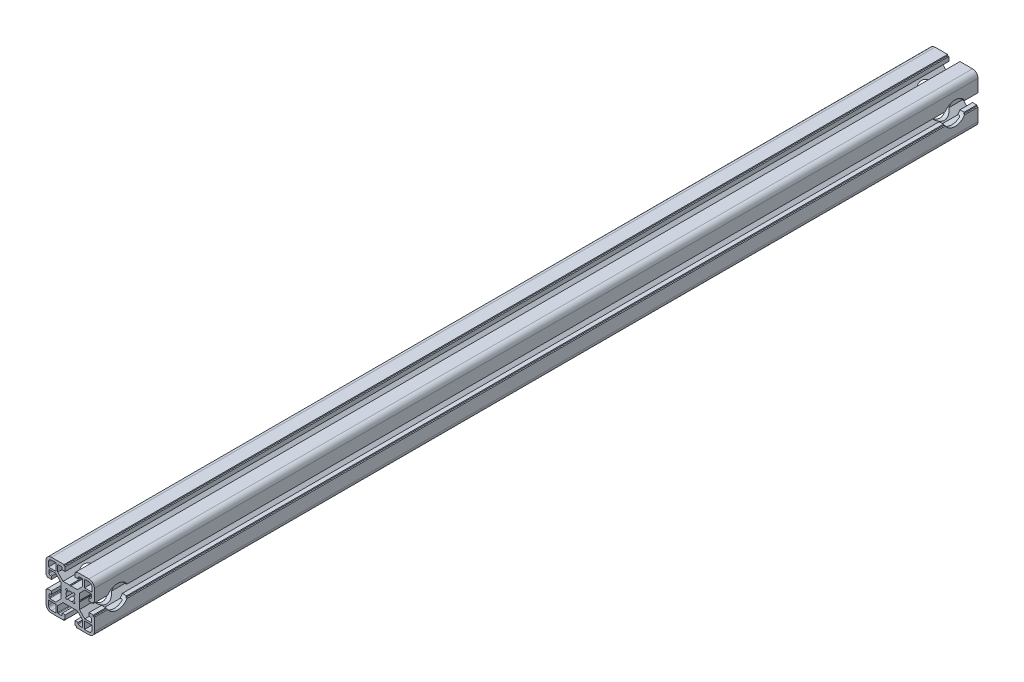
SolidWorks part; units mm, degrees
material "6061 GB/T6892-2006"
ref_plane "前视" through (0, 0, 0) normal (0, 0, 1) x (1, 0, 0)
ref_plane "上视" through (0, 0, 0) normal (0, 1, 0) x (1, 0, 0)
ref_plane "右视" through (0, 0, 0) normal (1, 0, 0) x (0, 0, -1)
sketch "草图1" plane through (0, 0, 0) normal (0, 0, 1) x (1, 0, 0)
  line L0 (-18.9995, -4.1003) -> (-18.9995, -5.1003)
  line L1 (-18.9995, -5.1003) -> (-19.9995, -5.1003)
  line L2 (-19.9995, -5.1003) -> (-19.9995, -15.5003)
  line L3 (-15.4995, -20.0003) -> (-5.0995, -20.0003)
  line L4 (-5.0995, -20.0003) -> (-5.0995, -19.0003)
  line L5 (-5.0995, -19.0003) -> (-4.0995, -19.0003)
  line L6 (-4.0995, -19.0003) -> (-4.0995, -15.5003)
  line L7 (-4.0995, -15.5003) -> (-6.5995, -15.5003)
  line L8 (-6.5995, -15.5003) -> (-6.5995, -16.5003)
  line L9 (-7.5995, -17.5003) -> (-9.7995, -17.5003)
  line L10 (-10.2995, -17.0003) -> (-10.2995, -11.9973)
  line L11 (-10.2995, -11.9973) -> (-5.9025, -7.6003)
  line L12 (-5.9025, -7.6003) -> (-0.5195, -7.6003)
  line L13 (-0.5195, -7.6003) -> (0.0005, -7.3003)
  line L14 (0.0005, -7.3003) -> (0.5195, -7.6003)
  line L15 (0.5195, -7.6003) -> (5.9035, -7.6003)
  line L16 (5.9035, -7.6003) -> (10.3005, -11.9973)
  line L17 (10.3005, -11.9973) -> (10.3005, -17.0003)
  line L18 (9.8005, -17.5003) -> (7.6005, -17.5003)
  line L19 (6.6005, -16.5003) -> (6.6005, -15.5003)
  line L20 (6.6005, -15.5003) -> (4.1005, -15.5003)
  line L21 (4.1005, -15.5003) -> (4.1005, -19.0003)
  line L22 (4.1005, -19.0003) -> (5.1005, -19.0003)
  line L23 (5.1005, -19.0003) -> (5.1005, -20.0003)
  line L24 (5.1005, -20.0003) -> (15.5005, -20.0003)
  line L25 (20.0005, -15.5003) -> (20.0005, -5.1003)
  line L26 (20.0005, -5.1003) -> (19.0005, -5.1003)
  line L27 (19.0005, -5.1003) -> (19.0005, -4.1003)
  line L28 (19.0005, -4.1003) -> (15.5005, -4.1003)
  line L29 (15.5005, -4.1003) -> (15.5005, -6.6003)
  line L30 (15.5005, -6.6003) -> (16.5005, -6.6003)
  line L31 (17.5005, -7.6003) -> (17.5005, -9.8003)
  line L32 (17.0005, -10.3003) -> (11.9975, -10.3003)
  line L33 (11.9975, -10.3003) -> (7.6005, -5.9033)
  line L34 (7.6005, -5.9033) -> (7.6005, -0.5203)
  line L35 (7.6005, -0.5203) -> (7.3005, -0.0003)
  line L36 (7.3005, -0.0003) -> (7.6005, 0.5197)
  line L37 (7.6005, 0.5197) -> (7.6005, 5.9027)
  line L38 (7.6005, 5.9027) -> (11.9975, 10.2997)
  line L39 (11.9975, 10.2997) -> (17.0005, 10.2997)
  line L40 (17.5005, 9.7997) -> (17.5005, 7.5997)
  line L41 (16.5005, 6.5997) -> (15.5005, 6.5997)
  line L42 (15.5005, 6.5997) -> (15.5005, 4.0997)
  line L43 (15.5005, 4.0997) -> (19.0005, 4.0997)
  line L44 (19.0005, 4.0997) -> (19.0005, 5.0997)
  line L45 (19.0005, 5.0997) -> (20.0005, 5.0997)
  line L46 (20.0005, 5.0997) -> (20.0005, 15.4997)
  line L47 (15.5005, 19.9997) -> (5.1005, 19.9997)
  line L48 (5.1005, 19.9997) -> (5.1005, 18.9997)
  line L49 (5.1005, 18.9997) -> (4.1005, 18.9997)
  line L50 (4.1005, 18.9997) -> (4.1005, 15.4997)
  line L51 (4.1005, 15.4997) -> (6.6005, 15.4997)
  line L52 (7.6005, 17.4997) -> (9.8005, 17.4997)
  line L53 (10.3005, 16.9997) -> (10.3005, 11.9967)
  line L54 (10.3005, 11.9967) -> (5.9035, 7.5997)
  line L55 (5.9035, 7.5997) -> (0.5195, 7.5997)
  line L56 (0.5195, 7.5997) -> (0.0005, 7.2997)
  line L57 (0.0005, 7.2997) -> (-0.5195, 7.5997)
  line L58 (-0.5195, 7.5997) -> (-5.9025, 7.5997)
  line L59 (-5.9025, 7.5997) -> (-10.2995, 11.9967)
  line L60 (-10.2995, 11.9967) -> (-10.2995, 16.9997)
  line L61 (-9.7995, 17.4997) -> (-7.5995, 17.4997)
  line L62 (-6.5995, 16.4997) -> (-6.5995, 15.4997)
  line L63 (-6.5995, 15.4997) -> (-4.0995, 15.4997)
  line L64 (-4.0995, 15.4997) -> (-4.0995, 18.9997)
  line L65 (-4.0995, 18.9997) -> (-5.0995, 18.9997)
  line L66 (-5.0995, 18.9997) -> (-5.0995, 19.9997)
  line L67 (-5.0995, 19.9997) -> (-15.4995, 19.9997)
  line L68 (-19.9995, 15.4997) -> (-19.9995, 5.0997)
  line L69 (-19.9995, 5.0997) -> (-18.9995, 5.0997)
  line L70 (-18.9995, 5.0997) -> (-18.9995, 4.0997)
  line L71 (-18.9995, 4.0997) -> (-15.4995, 4.0997)
  line L72 (-15.4995, 4.0997) -> (-15.4995, 6.5997)
  line L73 (-15.4995, 6.5997) -> (-16.4995, 6.5997)
  line L74 (-17.4995, 7.5997) -> (-17.4995, 9.7997)
  line L75 (-16.9995, 10.2997) -> (-11.9965, 10.2997)
  line L76 (-11.9965, 10.2997) -> (-7.5995, 5.9027)
  line L77 (-7.5995, 5.9027) -> (-7.5995, 0.5197)
  line L78 (-7.5995, 0.5197) -> (-7.2995, -0.0003)
  line L79 (-7.2995, -0.0003) -> (-7.5995, -0.5203)
  line L80 (-7.5995, -0.5203) -> (-7.5995, -5.9033)
  line L81 (-7.5995, -5.9033) -> (-11.9965, -10.3003)
  line L82 (-11.9965, -10.3003) -> (-16.9995, -10.3003)
  line L83 (-17.4995, -9.8003) -> (-17.4995, -7.6003)
  line L84 (-16.4995, -6.6003) -> (-15.4995, -6.6003)
  line L85 (-15.4995, -6.6003) -> (-15.4995, -4.1003)
  line L86 (-15.4995, -4.1003) -> (-18.9995, -4.1003)
  line L87 (15.5005, -18.0003) -> (11.8005, -18.0003)
  line L88 (11.8005, -18.0003) -> (11.8005, -11.8003)
  line L89 (11.8005, -11.8003) -> (18.0005, -11.8003)
  line L90 (18.0005, -11.8003) -> (18.0005, -15.5003)
  line L91 (18.0005, 11.7997) -> (11.8005, 11.7997)
  line L92 (11.8005, 11.7997) -> (11.8005, 17.9997)
  line L93 (11.8005, 17.9997) -> (15.5005, 17.9997)
  line L94 (18.0005, 15.4997) -> (18.0005, 11.7997)
  line L95 (-1.8145, -2.8753) -> (-3.0044, -4.0665)
  line L96 (-3.0044, -4.0665) -> (-4.0656, -3.0052)
  line L97 (-4.0656, -3.0052) -> (-2.8745, -1.8153)
  line L98 (-2.8745, 1.8147) -> (-4.0644, 3.0058)
  line L99 (-4.0644, 3.0058) -> (-3.0044, 4.0658)
  line L100 (-3.0044, 4.0658) -> (-1.8145, 2.8747)
  line L101 (1.8145, 2.8747) -> (3.0055, 4.0657)
  line L102 (3.0055, 4.0657) -> (4.0666, 3.0045)
  line L103 (4.0666, 3.0045) -> (2.8755, 1.8147)
  line L104 (2.8755, -1.8153) -> (4.0666, -3.0052)
  line L105 (4.0666, -3.0052) -> (3.0055, -4.0663)
  line L106 (3.0055, -4.0663) -> (1.8145, -2.8753)
  line L107 (-17.9995, -15.5003) -> (-17.9995, -11.8003)
  line L108 (-17.9995, -11.8003) -> (-11.7995, -11.8003)
  line L109 (-11.7995, -11.8003) -> (-11.7995, -18.0003)
  line L110 (-11.7995, -18.0003) -> (-15.4995, -18.0003)
  line L111 (-11.7995, 17.9997) -> (-11.7995, 11.7997)
  line L112 (-11.7995, 11.7997) -> (-17.9995, 11.7997)
  line L113 (-17.9995, 11.7997) -> (-17.9995, 15.4997)
  line L114 (-15.4995, 17.9997) -> (-11.7995, 17.9997)
  arc A0 (-19.9995, -15.5003) -> (-15.4995, -20.0003) centre (-15.4995, -15.5003) ccw
  arc A1 (-6.5995, -16.5003) -> (-7.5995, -17.5003) centre (-7.5995, -16.5003) cw
  arc A2 (-9.7995, -17.5003) -> (-10.2995, -17.0003) centre (-9.7995, -17.0003) cw
  arc A3 (10.3005, -17.0003) -> (9.8005, -17.5003) centre (9.8005, -17.0003) cw
  arc A4 (7.6005, -17.5003) -> (6.6005, -16.5003) centre (7.6005, -16.5003) cw
  arc A5 (15.5005, -20.0003) -> (20.0005, -15.5003) centre (15.5005, -15.5003) ccw
  arc A6 (16.5005, -6.6003) -> (17.5005, -7.6003) centre (16.5005, -7.6003) cw
  arc A7 (17.5005, -9.8003) -> (17.0005, -10.3003) centre (17.0005, -9.8003) cw
  arc A8 (17.0005, 10.2997) -> (17.5005, 9.7997) centre (17.0005, 9.7997) cw
  arc A9 (17.5005, 7.5997) -> (16.5005, 6.5997) centre (16.5005, 7.5997) cw
  arc A10 (20.0005, 15.4997) -> (15.5005, 19.9997) centre (15.5005, 15.4997) ccw
  arc A11 (6.6005, 15.4997) -> (6.6005, 16.4997) centre (7.1003, 15.9997) cw
  arc A12 (6.6005, 16.4997) -> (7.6005, 17.4997) centre (7.6005, 16.4997) cw
  arc A13 (9.8005, 17.4997) -> (10.3005, 16.9997) centre (9.8005, 16.9997) cw
  arc A14 (-10.2995, 16.9997) -> (-9.7995, 17.4997) centre (-9.7995, 16.9997) cw
  arc A15 (-7.5995, 17.4997) -> (-6.5995, 16.4997) centre (-7.5995, 16.4997) cw
  arc A16 (-15.4995, 19.9997) -> (-19.9995, 15.4997) centre (-15.4995, 15.4997) ccw
  arc A17 (-16.4995, 6.5997) -> (-17.4995, 7.5997) centre (-16.4995, 7.5997) cw
  arc A18 (-17.4995, 9.7997) -> (-16.9995, 10.2997) centre (-16.9995, 9.7997) cw
  arc A19 (-16.9995, -10.3003) -> (-17.4995, -9.8003) centre (-16.9995, -9.8003) cw
  arc A20 (-17.4995, -7.6003) -> (-16.4995, -6.6003) centre (-16.4995, -7.6003) cw
  arc A21 (18.0005, -15.5003) -> (15.5005, -18.0003) centre (15.5005, -15.5003) cw
  arc A22 (15.5005, 17.9997) -> (18.0005, 15.4997) centre (15.5005, 15.4997) cw
  arc A23 (-2.8745, -1.8153) -> (-2.8745, 1.8147) centre (0.0005, -0.0003) cw
  arc A24 (-1.8145, 2.8747) -> (1.8145, 2.8747) centre (0, -0.0007) cw
  arc A25 (2.8755, 1.8147) -> (2.8755, -1.8153) centre (0.0005, -0.0003) cw
  arc A26 (1.8145, -2.8753) -> (-1.8145, -2.8753) centre (0, 0) cw
  arc A27 (-15.4995, -18.0003) -> (-17.9995, -15.5003) centre (-15.4995, -15.5003) cw
  arc A28 (-17.9995, 15.4997) -> (-15.4995, 17.9997) centre (-15.4995, 15.4997) cw
extrude "凸台-拉伸1" add sketch "草图1" against normal blind 730
hole_wizard "Ø19.0 (19) 直径孔1" positions "草图2" profile "草图3" hole size "Ø19.0" standard "GB" end condition through all
sketch "草图2" plane through (-19.9995, -0.0008, 0) normal (1, 0, 0) x (0, -1, 0)
  line L2 (-0.0005, 730) -> (-0.0005, 0) construction
  point P0 (-0.0005, 19)
  point P4 (-0.0005, 711)
  dimension "D1" = 19
  dimension "D2" = 19
sketch "草图3" plane through (-19.9995, -0.0003, -19) normal (0, 1, 0) x (0, 0, 1)
  line L0 (0, 0) -> (0, 40)
  line L1 (0, 40) -> (9.5, 40)
  line L2 (9.5, 40) -> (9.5, 0)
  line L5 (9.5, 0) -> (0, 0)
  line L11 (0, -6.35) -> (0, 107.95) construction
  dimension "通孔孔直径" = 19
  dimension "通孔孔深度" = 40
